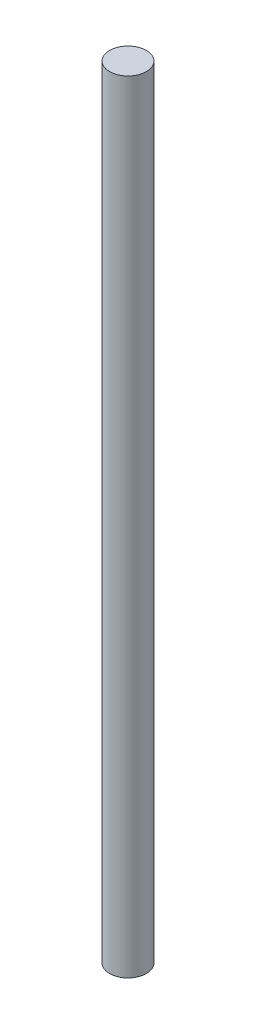
from build123d import *

# Parameters (mm, degrees)
SKETCH1_R           = 2
BOSS_EXTRUDE1_DEPTH = 85


with BuildPart() as part:
    # Sketch1 → Boss-Extrude1 (new body)
    with BuildSketch(Plane(origin=(0, 0, 0), x_dir=(1, 0, 0), z_dir=(0, 1, 0))):
        with Locations(Location((0, 0, 0), (0, 0, 270))):
            Circle(SKETCH1_R)
    extrude(amount=BOSS_EXTRUDE1_DEPTH)


solid = part.part
